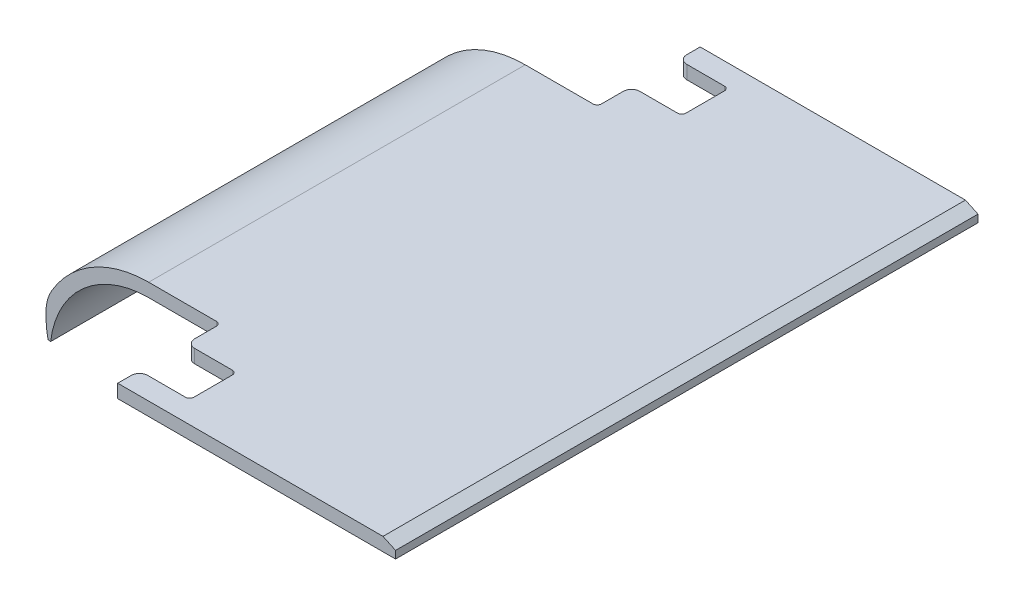
SolidWorks part; units mm, degrees
material "普通碳钢"
ref_plane "Front Plane" through (0, 0, 0) normal (0, 0, 1) x (1, 0, 0)
ref_plane "Top Plane" through (0, 0, 0) normal (0, 1, 0) x (1, 0, 0)
ref_plane "Right Plane" through (0, 0, 0) normal (1, 0, 0) x (0, 0, -1)
sketch "Sketch1" plane through (0, 0, 0) normal (0, 0, 1) x (1, 0, 0)
  line L0 (0, 0) -> (418, 0)
  line L1 (418, 0) -> (418, 9)
  line L2 (418, 9) -> (403, 16)
  line L3 (0, -66) -> (0, 66) construction
  line L4 (-117.1665, -104) -> (-133.0535, -102.1017)
  line L5 (0, 16) -> (403, 16)
  arc A0 (0, 16) -> (-133.0535, -102.1017) centre (0, -118) ccw
  arc A1 (0, 0) -> (-117.1665, -104) centre (0, -118) ccw
  arc A3 (0, 16) -> (-133.0535, -102.1017) centre (0, -118) ccw construction
  point P1 (304.9758, 15.801)
  point P3 (968.8866, -12.7147)
  point P4 (306.2556, 15.7461)
  point P9 (968.8866, -12.7147)
  point P12 (497.7056, -4000)
  point P15 (817.474, 3.2492)
  dimension "D3" = 15
  dimension "D1" = 9
  dimension "D4" = 118
  dimension "D2" = 16
  dimension "D5" = 418
  dimension "D6" = 104
extrude "Boss-Extrude1" add sketch "Sketch1" along normal mid plane 696
sketch "Sketch2" plane through (0, 0, 0) normal (0, 1, 0) x (1, 0, 0)
  line L0 (86, -256) -> (86, -230)
  line L2 (96, 322) -> (141, 322)
  line L3 (146, 317) -> (146, 271)
  line L4 (141, 266) -> (96, 266)
  line L5 (86, 256) -> (86, 230)
  line L6 (81, 225) -> (-133.0535, 225)
  line L7 (86, 332) -> (86, 348)
  line L8 (86, 348) -> (-133.0535, 348)
  line L9 (0, 348) -> (-133.0535, 348) construction
  line L10 (86, -332) -> (86, -348)
  line L11 (86, -348) -> (-133.0535, -348)
  line L12 (81, -225) -> (-133.0535, -225)
  line L13 (418, -348) -> (418, 348) construction
  line L14 (141, -266) -> (96, -266)
  line L15 (146, -317) -> (146, -271)
  line L16 (-133.0535, -348) -> (-133.0535, -225)
  line L17 (96, -322) -> (141, -322)
  line L20 (-133.0535, 348) -> (-133.0535, 225)
  line L21 (418, 0) -> (-96.7747, 0) construction
  line L22 (418, -348) -> (418, 348) construction
  line L23 (-133.0535, -348) -> (-133.0535, 348) construction
  arc A0 (96, 266) -> (86, 256) centre (96, 256) ccw
  arc A1 (96, 322) -> (86, 332) centre (96, 332) cw
  arc A2 (86, 230) -> (81, 225) centre (81, 230) cw
  arc A3 (141, 266) -> (146, 271) centre (141, 271) ccw
  arc A4 (146, 317) -> (141, 322) centre (141, 317) ccw
  arc A5 (86, -230) -> (81, -225) centre (81, -230) ccw
  arc A7 (146, -317) -> (141, -322) centre (141, -317) cw
  arc A8 (141, -266) -> (146, -271) centre (141, -271) cw
  arc A10 (96, -322) -> (86, -332) centre (96, -332) ccw
  arc A11 (96, -266) -> (86, -256) centre (96, -256) cw
  dimension "D3" = 10
  dimension "D4" = 5
  dimension "D5" = 644
  dimension "D1" = 450
  dimension "D8" = 10
  dimension "D2" = 532
  dimension "D6" = 332
  dimension "D7" = 60
extrude "Cut-Extrude1" cut sketch "Sketch2" against normal through all and the other way through all
sketch "Sketch3" plane through (0, 0, 225) normal (0, 0, 1) x (1, 0, 0)
  line L0 (0, -66) -> (0, 66) construction
  line L1 (81, 0) -> (0, 0) construction
  line L2 (-117.1665, -104) -> (-133.0535, -102.1017) construction
  line L3 (-120.3057, -103.6249) -> (-133.0535, -102.1017)
  arc A0 (-122.6947, -73.9145) -> (-120.3057, -103.6249) centre (0, -79) ccw
  arc A1 (0, 16) -> (-133.0535, -102.1017) centre (0, -118) ccw construction
  arc A2 (-116.0337, -50.9763) -> (-133.0535, -102.1017) centre (0, -118) ccw
  arc A3 (-116.0337, -50.9763) -> (-122.6947, -73.9145) centre (-72.7375, -75.9851) ccw
  point P8 (40.5, 0)
  dimension "D1" = 122.8
  dimension "D3" = 50
  dimension "D2" = 79
extrude "Cut-Extrude3" cut sketch "Sketch3" against normal through all
